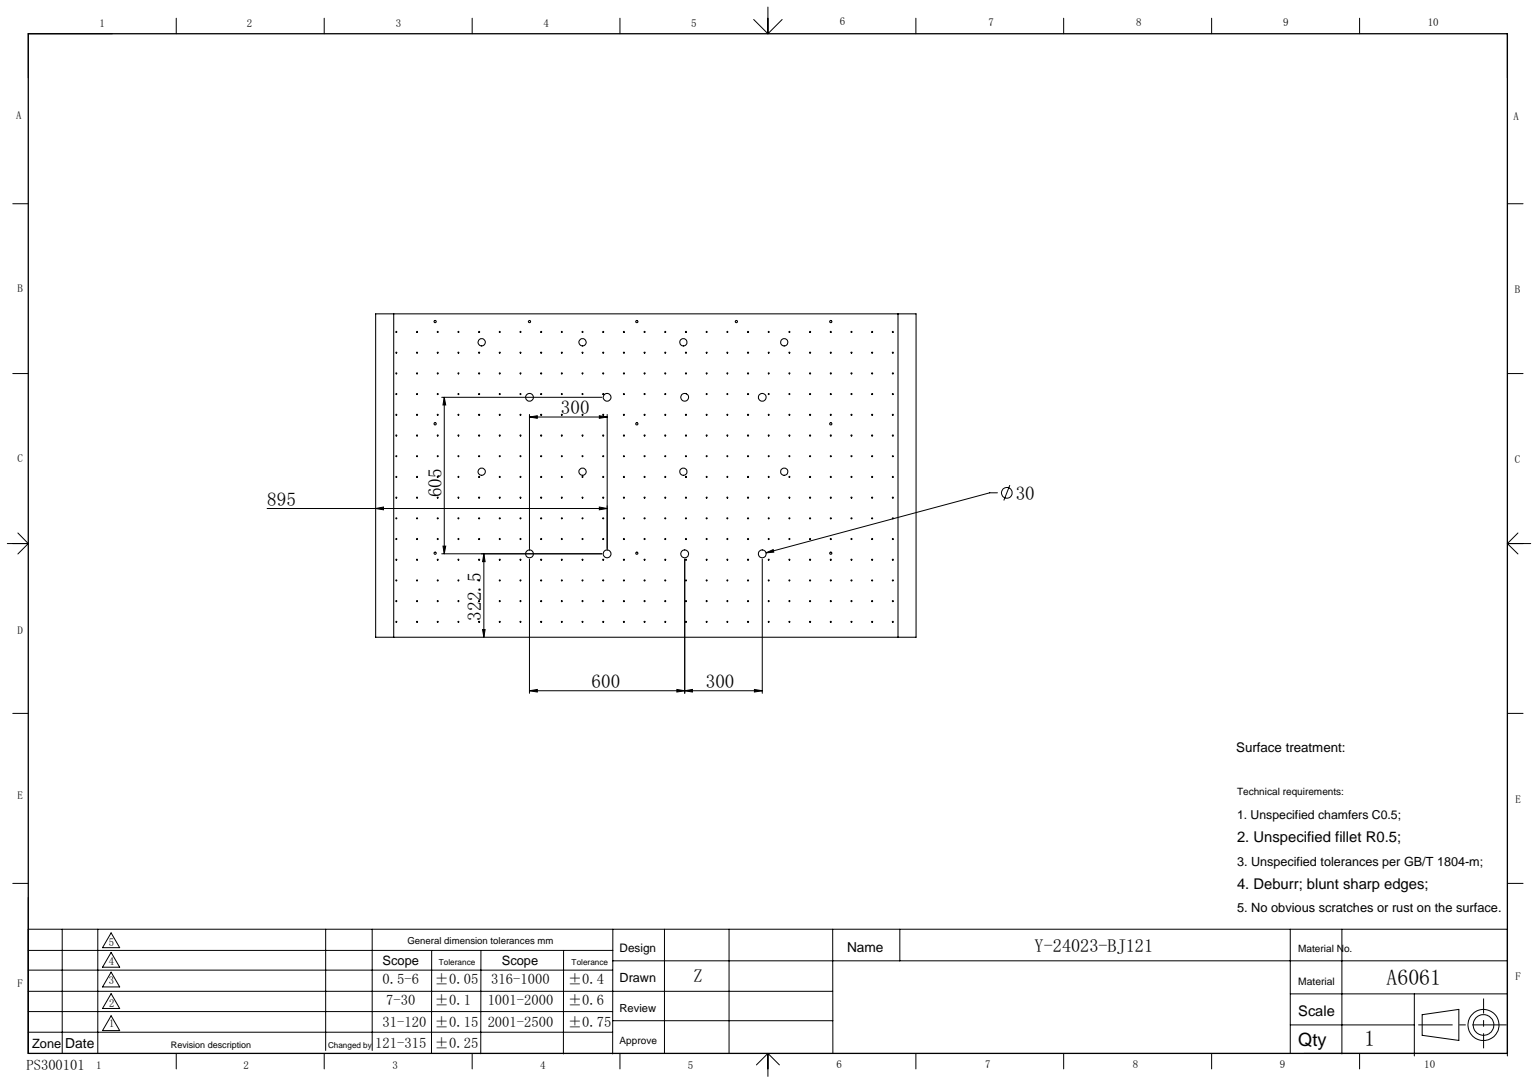
SolidWorks part; units mm, degrees
material "A6061"
ref_plane "前基準面" through (0, 0, 0) normal (0, 0, 1) x (1, 0, 0)
ref_plane "上基準面" through (0, 0, 0) normal (0, 1, 0) x (1, 0, 0)
ref_plane "右基準面" through (0, 0, 0) normal (1, 0, 0) x (0, 0, -1)
sketch "草图1" plane through (0, 0, 0) normal (0, 1, 0) x (1, 0, 0)
  line L1 (-1095, -675) -> (1095, -675)
  line L2 (-1095, -675) -> (-1095, 675)
  line L3 (-1095, 675) -> (1095, 675)
  line L4 (1095, -675) -> (1095, 675)
  line L5 (-1095, -675) -> (1095, 675) construction
  line L6 (-1095, 675) -> (1095, -675) construction
  point P0 (0, 0)
  dimension "D1" = 2190
  dimension "D2" = 1350
extrude "凸台-拉伸1" add sketch "草图1" along normal mid plane 2
hole_wizard "Ø25.0 (25) 直径孔1" positions "草图6" profile "草图7" hole size "Ø25.0" standard "GB" end condition through all
sketch "草图6" plane through (0, 1, 0) normal (0, 1, 0) x (1, 0, 0)
  line L0 (0, 787.4627) -> (0, 0) construction
  line L2 (1095, 675) -> (-1095, 675) construction
  point P0 (-585, 565)
  point P5 (-195, 565)
  point P6 (195, 565)
  point P7 (585, 565)
  point P20 (-585, 65)
  point P21 (-195, 65)
  point P22 (195, 65)
  point P23 (585, 65)
  dimension "D2" = 390
  dimension "D3" = 110
  dimension "D5" = 500
  dimension "D1" = 4
  dimension "D4" = 2
sketch "草图7" plane through (-585, 1, -565) normal (1, 0, 0) x (0, 0, 1)
  line L0 (0, 0) -> (0, 2)
  line L1 (0, 2) -> (14, 2)
  line L2 (14, 2) -> (14, 0)
  line L5 (14, 0) -> (0, 0)
  line L11 (0, -6.35) -> (0, 107.95) construction
  dimension "通孔孔直径" = 28
  dimension "通孔孔深度" = 2
hole_wizard "M6 锥坑高头螺钉的锥形沉头孔1" positions "草图10" profile "草图11" countersink size "M6" standard "ISO" end condition through all
sketch "草图10" plane through (0, -1, 0) normal (0, -1, 0) x (-1, 0, 0)
  line L0 (0, 877.4584) -> (0, 0) construction
  line L1 (0, 0) -> (-1346.5612, 0) construction
  line L3 (-1095, -675) -> (-1095, 675) construction
  line L4 (-1095, 675) -> (1095, 675) construction
  point P0 (-765, 645)
  point P2 (-400, 645)
  point P4 (-765, 250)
  point P18 (765, 250)
  point P19 (400, 645)
  point P20 (765, 645)
  point P21 (765, -645)
  point P22 (400, -645)
  point P23 (765, -250)
  point P26 (-765, -250)
  point P27 (-400, -645)
  point P28 (-765, -645)
  point P37 (-15, -645)
  point P38 (-15, -250)
  point P39 (-15, 250)
  point P40 (-15, 645)
  point P46 (1075, 250)
  point P47 (1075, 645)
  point P48 (1075, -645)
  point P49 (1075, -250)
  point P52 (-1075, 645)
  point P53 (-1075, 250)
  point P54 (-1075, -250)
  point P55 (-1075, -645)
  dimension "D1" = 800
  dimension "D2" = 330
  dimension "D3" = 30
  dimension "D4" = 500
  dimension "D5" = 2
  dimension "D6" = 2
sketch "草图11" plane through (765, -1, -645) normal (1, 0, 0) x (0, 0, -1)
  line L0 (0, 0) -> (0, 2)
  line L1 (0, 2) -> (3.3, 2)
  line L2 (3.3, 2) -> (3.3, 3)
  line L3 (3.3, 3) -> (6.3, 0)
  line L5 (6.3, 0) -> (0, 0)
  line L6 (-3.3, 3) -> (-6.3, 0) construction
  line L11 (0, -6.35) -> (0, 107.95) construction
  dimension "通孔孔直径" = 6.6
  dimension "通孔孔深度" = 2
  dimension "近端锥形沉头孔直径" = 12.6
  dimension "近端锥形沉头孔角度" = 90
fillet "圆角1" radius 10 4 edges at (1095, 0, -675) (-1095, 0, -675) (-1095, 0, 675) (1095, 0, 675)
sketch "草图12" plane through (0, 1, 0) normal (0, 1, 0) x (1, 0, 0)
  line L1 (-985, -575) -> (1222.9953, -575)
  line L2 (1222.9953, -575) -> (1222.9953, -1049.3537)
  line L3 (1222.9953, -1049.3537) -> (-995, -1049.3537)
  line L7 (-1085, -675) -> (1085, -675) construction
  line L9 (-995, -565) -> (-995, 792.5095)
  line L10 (-995, 792.5095) -> (-1180.58, 792.5095)
  line L11 (-1180.58, 792.5095) -> (-1180.58, -1049.3537)
  line L12 (-1180.58, -1049.3537) -> (-995, -1049.3537)
  line L13 (-1095, 665) -> (-1095, -665) construction
  arc A0 (-995, -565) -> (-985, -575) centre (-985, -565) ccw
  dimension "D3" = 10
  dimension "D1" = 100
  dimension "D2" = 100
extrude "切除-拉伸1" cut sketch "草图12" against normal blind 10
fillet "圆角2" radius 5 2 edges at (1095, 0, 575) (-995, 0, -675)
sketch "草图13" plane through (0, 1, 0) normal (0, 1, 0) x (1, 0, 0)
  line L0 (-995, -565) -> (-995, 670) construction
  line L1 (1090, -575) -> (-985, -575) construction
  circle A0 centre (-915, -515) radius 2
  circle A1 centre (-835, -515) radius 2
  circle A2 centre (-755, -515) radius 2
  circle A3 centre (-675, -515) radius 2
  circle A4 centre (-595, -515) radius 2
  circle A5 centre (-515, -515) radius 2
  circle A6 centre (-435, -515) radius 2
  circle A7 centre (-355, -515) radius 2
  circle A8 centre (-275, -515) radius 2
  circle A9 centre (-195, -515) radius 2
  circle A10 centre (-115, -515) radius 2
  circle A11 centre (-35, -515) radius 2
  circle A12 centre (45, -515) radius 2
  circle A13 centre (125, -515) radius 2
  circle A14 centre (205, -515) radius 2
  circle A15 centre (285, -515) radius 2
  circle A16 centre (365, -515) radius 2
  circle A17 centre (445, -515) radius 2
  circle A18 centre (525, -515) radius 2
  circle A19 centre (605, -515) radius 2
  circle A20 centre (685, -515) radius 2
  circle A21 centre (765, -515) radius 2
  circle A22 centre (845, -515) radius 2
  circle A23 centre (925, -515) radius 2
  circle A24 centre (1005, -515) radius 2
  circle A33 centre (-835, -435) radius 2
  circle A34 centre (-755, -435) radius 2
  circle A35 centre (-675, -435) radius 2
  circle A36 centre (-595, -435) radius 2
  circle A37 centre (-515, -435) radius 2
  circle A38 centre (-435, -435) radius 2
  circle A39 centre (-355, -435) radius 2
  circle A40 centre (-275, -435) radius 2
  circle A41 centre (-195, -435) radius 2
  circle A42 centre (-115, -435) radius 2
  circle A43 centre (-35, -435) radius 2
  circle A44 centre (45, -435) radius 2
  circle A45 centre (125, -435) radius 2
  circle A46 centre (205, -435) radius 2
  circle A47 centre (285, -435) radius 2
  circle A48 centre (365, -435) radius 2
  circle A49 centre (445, -435) radius 2
  circle A50 centre (525, -435) radius 2
  circle A51 centre (605, -435) radius 2
  circle A52 centre (685, -435) radius 2
  circle A53 centre (765, -435) radius 2
  circle A54 centre (845, -435) radius 2
  circle A55 centre (925, -435) radius 2
  circle A56 centre (1005, -435) radius 2
  circle A65 centre (-835, -355) radius 2
  circle A66 centre (-755, -355) radius 2
  circle A67 centre (-675, -355) radius 2
  circle A68 centre (-595, -355) radius 2
  circle A69 centre (-515, -355) radius 2
  circle A70 centre (-435, -355) radius 2
  circle A71 centre (-355, -355) radius 2
  circle A72 centre (-275, -355) radius 2
  circle A73 centre (-195, -355) radius 2
  circle A74 centre (-115, -355) radius 2
  circle A75 centre (-35, -355) radius 2
  circle A76 centre (45, -355) radius 2
  circle A77 centre (125, -355) radius 2
  circle A78 centre (205, -355) radius 2
  circle A79 centre (285, -355) radius 2
  circle A80 centre (365, -355) radius 2
  circle A81 centre (445, -355) radius 2
  circle A82 centre (525, -355) radius 2
  circle A83 centre (605, -355) radius 2
  circle A84 centre (685, -355) radius 2
  circle A85 centre (765, -355) radius 2
  circle A86 centre (845, -355) radius 2
  circle A87 centre (925, -355) radius 2
  circle A88 centre (1005, -355) radius 2
  circle A97 centre (-835, -275) radius 2
  circle A98 centre (-755, -275) radius 2
  circle A99 centre (-675, -275) radius 2
  circle A100 centre (-595, -275) radius 2
  circle A101 centre (-515, -275) radius 2
  circle A102 centre (-435, -275) radius 2
  circle A103 centre (-355, -275) radius 2
  circle A104 centre (-275, -275) radius 2
  circle A105 centre (-195, -275) radius 2
  circle A106 centre (-115, -275) radius 2
  circle A107 centre (-35, -275) radius 2
  circle A108 centre (45, -275) radius 2
  circle A109 centre (125, -275) radius 2
  circle A110 centre (205, -275) radius 2
  circle A111 centre (285, -275) radius 2
  circle A112 centre (365, -275) radius 2
  circle A113 centre (445, -275) radius 2
  circle A114 centre (525, -275) radius 2
  circle A115 centre (605, -275) radius 2
  circle A116 centre (685, -275) radius 2
  circle A117 centre (765, -275) radius 2
  circle A118 centre (845, -275) radius 2
  circle A119 centre (925, -275) radius 2
  circle A120 centre (1005, -275) radius 2
  circle A129 centre (-835, -195) radius 2
  circle A130 centre (-755, -195) radius 2
  circle A131 centre (-675, -195) radius 2
  circle A132 centre (-595, -195) radius 2
  circle A133 centre (-515, -195) radius 2
  circle A134 centre (-435, -195) radius 2
  circle A135 centre (-355, -195) radius 2
  circle A136 centre (-275, -195) radius 2
  circle A137 centre (-195, -195) radius 2
  circle A138 centre (-115, -195) radius 2
  circle A139 centre (-35, -195) radius 2
  circle A140 centre (45, -195) radius 2
  circle A141 centre (125, -195) radius 2
  circle A142 centre (205, -195) radius 2
  circle A143 centre (285, -195) radius 2
  circle A144 centre (365, -195) radius 2
  circle A145 centre (445, -195) radius 2
  circle A146 centre (525, -195) radius 2
  circle A147 centre (605, -195) radius 2
  circle A148 centre (685, -195) radius 2
  circle A149 centre (765, -195) radius 2
  circle A150 centre (845, -195) radius 2
  circle A151 centre (925, -195) radius 2
  circle A152 centre (1005, -195) radius 2
  circle A161 centre (-835, -115) radius 2
  circle A162 centre (-755, -115) radius 2
  circle A163 centre (-675, -115) radius 2
  circle A164 centre (-595, -115) radius 2
  circle A165 centre (-515, -115) radius 2
  circle A166 centre (-435, -115) radius 2
  circle A167 centre (-355, -115) radius 2
  circle A168 centre (-275, -115) radius 2
  circle A169 centre (-195, -115) radius 2
  circle A170 centre (-115, -115) radius 2
  circle A171 centre (-35, -115) radius 2
  circle A172 centre (45, -115) radius 2
  circle A173 centre (125, -115) radius 2
  circle A174 centre (205, -115) radius 2
  circle A175 centre (285, -115) radius 2
  circle A176 centre (365, -115) radius 2
  circle A177 centre (445, -115) radius 2
  circle A178 centre (525, -115) radius 2
  circle A179 centre (605, -115) radius 2
  circle A180 centre (685, -115) radius 2
  circle A181 centre (765, -115) radius 2
  circle A182 centre (845, -115) radius 2
  circle A183 centre (925, -115) radius 2
  circle A184 centre (1005, -115) radius 2
  circle A193 centre (-835, -35) radius 2
  circle A194 centre (-755, -35) radius 2
  circle A195 centre (-675, -35) radius 2
  circle A196 centre (-595, -35) radius 2
  circle A197 centre (-515, -35) radius 2
  circle A198 centre (-435, -35) radius 2
  circle A199 centre (-355, -35) radius 2
  circle A200 centre (-275, -35) radius 2
  circle A201 centre (-195, -35) radius 2
  circle A202 centre (-115, -35) radius 2
  circle A203 centre (-35, -35) radius 2
  circle A204 centre (45, -35) radius 2
  circle A205 centre (125, -35) radius 2
  circle A206 centre (205, -35) radius 2
  circle A207 centre (285, -35) radius 2
  circle A208 centre (365, -35) radius 2
  circle A209 centre (445, -35) radius 2
  circle A210 centre (525, -35) radius 2
  circle A211 centre (605, -35) radius 2
  circle A212 centre (685, -35) radius 2
  circle A213 centre (765, -35) radius 2
  circle A214 centre (845, -35) radius 2
  circle A215 centre (925, -35) radius 2
  circle A216 centre (1005, -35) radius 2
  circle A225 centre (-835, 45) radius 2
  circle A226 centre (-755, 45) radius 2
  circle A227 centre (-675, 45) radius 2
  circle A228 centre (-595, 45) radius 2
  circle A229 centre (-515, 45) radius 2
  circle A230 centre (-435, 45) radius 2
  circle A231 centre (-355, 45) radius 2
  circle A232 centre (-275, 45) radius 2
  circle A233 centre (-195, 45) radius 2
  circle A234 centre (-115, 45) radius 2
  circle A235 centre (-35, 45) radius 2
  circle A236 centre (45, 45) radius 2
  circle A237 centre (125, 45) radius 2
  circle A238 centre (205, 45) radius 2
  circle A239 centre (285, 45) radius 2
  circle A240 centre (365, 45) radius 2
  circle A241 centre (445, 45) radius 2
  circle A242 centre (525, 45) radius 2
  circle A243 centre (605, 45) radius 2
  circle A244 centre (685, 45) radius 2
  circle A245 centre (765, 45) radius 2
  circle A246 centre (845, 45) radius 2
  circle A247 centre (925, 45) radius 2
  circle A248 centre (1005, 45) radius 2
  circle A257 centre (-835, 125) radius 2
  circle A258 centre (-755, 125) radius 2
  circle A259 centre (-675, 125) radius 2
  circle A260 centre (-595, 125) radius 2
  circle A261 centre (-515, 125) radius 2
  circle A262 centre (-435, 125) radius 2
  circle A263 centre (-355, 125) radius 2
  circle A264 centre (-275, 125) radius 2
  circle A265 centre (-195, 125) radius 2
  circle A266 centre (-115, 125) radius 2
  circle A267 centre (-35, 125) radius 2
  circle A268 centre (45, 125) radius 2
  circle A269 centre (125, 125) radius 2
  circle A270 centre (205, 125) radius 2
  circle A271 centre (285, 125) radius 2
  circle A272 centre (365, 125) radius 2
  circle A273 centre (445, 125) radius 2
  circle A274 centre (525, 125) radius 2
  circle A275 centre (605, 125) radius 2
  circle A276 centre (685, 125) radius 2
  circle A277 centre (765, 125) radius 2
  circle A278 centre (845, 125) radius 2
  circle A279 centre (925, 125) radius 2
  circle A280 centre (1005, 125) radius 2
  circle A289 centre (-835, 205) radius 2
  circle A290 centre (-755, 205) radius 2
  circle A291 centre (-675, 205) radius 2
  circle A292 centre (-595, 205) radius 2
  circle A293 centre (-515, 205) radius 2
  circle A294 centre (-435, 205) radius 2
  circle A295 centre (-355, 205) radius 2
  circle A296 centre (-275, 205) radius 2
  circle A297 centre (-195, 205) radius 2
  circle A298 centre (-115, 205) radius 2
  circle A299 centre (-35, 205) radius 2
  circle A300 centre (45, 205) radius 2
  circle A301 centre (125, 205) radius 2
  circle A302 centre (205, 205) radius 2
  circle A303 centre (285, 205) radius 2
  circle A304 centre (365, 205) radius 2
  circle A305 centre (445, 205) radius 2
  circle A306 centre (525, 205) radius 2
  circle A307 centre (605, 205) radius 2
  circle A308 centre (685, 205) radius 2
  circle A309 centre (765, 205) radius 2
  circle A310 centre (845, 205) radius 2
  circle A311 centre (925, 205) radius 2
  circle A312 centre (1005, 205) radius 2
  circle A321 centre (-835, 285) radius 2
  circle A322 centre (-755, 285) radius 2
  circle A323 centre (-675, 285) radius 2
  circle A324 centre (-595, 285) radius 2
  circle A325 centre (-515, 285) radius 2
  circle A326 centre (-435, 285) radius 2
  circle A327 centre (-355, 285) radius 2
  circle A328 centre (-275, 285) radius 2
  circle A329 centre (-195, 285) radius 2
  circle A330 centre (-115, 285) radius 2
  circle A331 centre (-35, 285) radius 2
  circle A332 centre (45, 285) radius 2
  circle A333 centre (125, 285) radius 2
  circle A334 centre (205, 285) radius 2
  circle A335 centre (285, 285) radius 2
  circle A336 centre (365, 285) radius 2
  circle A337 centre (445, 285) radius 2
  circle A338 centre (525, 285) radius 2
  circle A339 centre (605, 285) radius 2
  circle A340 centre (685, 285) radius 2
  circle A341 centre (765, 285) radius 2
  circle A342 centre (845, 285) radius 2
  circle A343 centre (925, 285) radius 2
  circle A344 centre (1005, 285) radius 2
  circle A353 centre (-835, 365) radius 2
  circle A354 centre (-755, 365) radius 2
  circle A355 centre (-675, 365) radius 2
  circle A356 centre (-595, 365) radius 2
  circle A357 centre (-515, 365) radius 2
  circle A358 centre (-435, 365) radius 2
  circle A359 centre (-355, 365) radius 2
  circle A360 centre (-275, 365) radius 2
  circle A361 centre (-195, 365) radius 2
  circle A362 centre (-115, 365) radius 2
  circle A363 centre (-35, 365) radius 2
  circle A364 centre (45, 365) radius 2
  circle A365 centre (125, 365) radius 2
  circle A366 centre (205, 365) radius 2
  circle A367 centre (285, 365) radius 2
  circle A368 centre (365, 365) radius 2
  circle A369 centre (445, 365) radius 2
  circle A370 centre (525, 365) radius 2
  circle A371 centre (605, 365) radius 2
  circle A372 centre (685, 365) radius 2
  circle A373 centre (765, 365) radius 2
  circle A374 centre (845, 365) radius 2
  circle A375 centre (925, 365) radius 2
  circle A376 centre (1005, 365) radius 2
  circle A385 centre (-835, 445) radius 2
  circle A386 centre (-755, 445) radius 2
  circle A387 centre (-675, 445) radius 2
  circle A388 centre (-595, 445) radius 2
  circle A389 centre (-515, 445) radius 2
  circle A390 centre (-435, 445) radius 2
  circle A391 centre (-355, 445) radius 2
  circle A392 centre (-275, 445) radius 2
  circle A393 centre (-195, 445) radius 2
  circle A394 centre (-115, 445) radius 2
  circle A395 centre (-35, 445) radius 2
  circle A396 centre (45, 445) radius 2
  circle A397 centre (125, 445) radius 2
  circle A398 centre (205, 445) radius 2
  circle A399 centre (285, 445) radius 2
  circle A400 centre (365, 445) radius 2
  circle A401 centre (445, 445) radius 2
  circle A402 centre (525, 445) radius 2
  circle A403 centre (605, 445) radius 2
  circle A404 centre (685, 445) radius 2
  circle A405 centre (765, 445) radius 2
  circle A406 centre (845, 445) radius 2
  circle A407 centre (925, 445) radius 2
  circle A408 centre (1005, 445) radius 2
  circle A417 centre (-835, 525) radius 2
  circle A418 centre (-755, 525) radius 2
  circle A419 centre (-675, 525) radius 2
  circle A420 centre (-595, 525) radius 2
  circle A421 centre (-515, 525) radius 2
  circle A422 centre (-435, 525) radius 2
  circle A423 centre (-355, 525) radius 2
  circle A424 centre (-275, 525) radius 2
  circle A425 centre (-195, 525) radius 2
  circle A426 centre (-115, 525) radius 2
  circle A427 centre (-35, 525) radius 2
  circle A428 centre (45, 525) radius 2
  circle A429 centre (125, 525) radius 2
  circle A430 centre (205, 525) radius 2
  circle A431 centre (285, 525) radius 2
  circle A432 centre (365, 525) radius 2
  circle A433 centre (445, 525) radius 2
  circle A434 centre (525, 525) radius 2
  circle A435 centre (605, 525) radius 2
  circle A436 centre (685, 525) radius 2
  circle A437 centre (765, 525) radius 2
  circle A438 centre (845, 525) radius 2
  circle A439 centre (925, 525) radius 2
  circle A440 centre (1005, 525) radius 2
  circle A449 centre (-835, 605) radius 2
  circle A450 centre (-755, 605) radius 2
  circle A451 centre (-675, 605) radius 2
  circle A452 centre (-595, 605) radius 2
  circle A453 centre (-515, 605) radius 2
  circle A454 centre (-435, 605) radius 2
  circle A455 centre (-355, 605) radius 2
  circle A456 centre (-275, 605) radius 2
  circle A457 centre (-195, 605) radius 2
  circle A458 centre (-115, 605) radius 2
  circle A459 centre (-35, 605) radius 2
  circle A460 centre (45, 605) radius 2
  circle A461 centre (125, 605) radius 2
  circle A462 centre (205, 605) radius 2
  circle A463 centre (285, 605) radius 2
  circle A464 centre (365, 605) radius 2
  circle A465 centre (445, 605) radius 2
  circle A466 centre (525, 605) radius 2
  circle A467 centre (605, 605) radius 2
  circle A468 centre (685, 605) radius 2
  circle A469 centre (765, 605) radius 2
  circle A470 centre (845, 605) radius 2
  circle A471 centre (925, 605) radius 2
  circle A472 centre (1005, 605) radius 2
  circle A641 centre (-915, -435) radius 2
  circle A642 centre (-915, -355) radius 2
  circle A643 centre (-915, -275) radius 2
  circle A644 centre (-915, -195) radius 2
  circle A645 centre (-915, -115) radius 2
  circle A646 centre (-915, -35) radius 2
  circle A647 centre (-915, 45) radius 2
  circle A648 centre (-915, 125) radius 2
  circle A649 centre (-915, 205) radius 2
  circle A650 centre (-915, 285) radius 2
  circle A651 centre (-915, 365) radius 2
  circle A652 centre (-915, 445) radius 2
  circle A653 centre (-915, 525) radius 2
  circle A654 centre (-915, 605) radius 2
  dimension "D1" = 4
  dimension "D2" = 80
  dimension "D5" = 60
  dimension "D3" = 25
  dimension "D4" = 15
extrude "切除-拉伸2" cut sketch "草图13" against normal blind 10
sketch "草图14" plane through (0, 1, 0) normal (0, 1, 0) x (1, 0, 0)
  line L0 (1090, -575) -> (-985, -575) construction
  line L1 (-995, 675) -> (-925, 675)
  line L2 (-995, 675) -> (-995, -575)
  line L3 (-995, -575) -> (-925, -575)
  line L4 (-925, 675) -> (-925, -575)
  line L5 (0, 0) -> (0, -165.5843) construction
  line L6 (1085, 675) -> (-990, 675) construction
  line L7 (1095, -575) -> (1025, -575)
  line L8 (1095, -575) -> (1095, 675)
  line L9 (1095, 675) -> (1025, 675)
  line L10 (1025, -575) -> (1025, 675)
  line L11 (1095, -570) -> (1095, 665) construction
  line L12 (-995, -565) -> (-995, 670) construction
  dimension "D1" = 70
  dimension "D2" = 70
extrude "凸台-拉伸2" add sketch "草图14" along normal mid plane 1 separate body
hole_wizard "Ø20.0 (30) 直径孔1" positions "草图16" profile "草图15" hole size "Ø20.0" standard "ISO"
sketch "草图16" plane through (0, -1, 0) normal (0, -1, 0) x (-1, 0, 0)
  line L0 (400, -252.5) -> (100, -252.5) construction
  line L1 (400, 352.5) -> (100, 352.5) construction
  line L2 (100, 352.5) -> (100, -252.5) construction
  circle A0 centre (400, 352.5) radius 5.5 construction
  circle A1 centre (-500, 352.5) radius 5.5 construction
  circle A2 centre (-200, 352.5) radius 5.5 construction
  circle A3 centre (400, -252.5) radius 5.5 construction
  circle A4 centre (-500, -252.5) radius 5.5 construction
  circle A5 centre (-200, -252.5) radius 5.5 construction
  point P0 (400, 352.5)
  point P1 (-500, 352.5)
  point P2 (-200, 352.5)
  point P3 (400, -252.5)
  point P4 (-500, -252.5)
  point P5 (-200, -252.5)
  point P19 (100, -252.5)
  point P28 (100, 352.5)
  dimension "D1" = 300
sketch "草图15" plane through (-400, -1, -352.5) normal (1, 0, 0) x (0, 0, -1)
  line L0 (0, 0) -> (0, 2)
  line L1 (0, 2) -> (15, 2)
  line L2 (15, 2) -> (15, 0)
  line L5 (15, 0) -> (0, 0)
  line L11 (0, -6.35) -> (0, 107.95) construction
  dimension "通孔孔直径" = 30
  dimension "通孔孔深度" = 2
